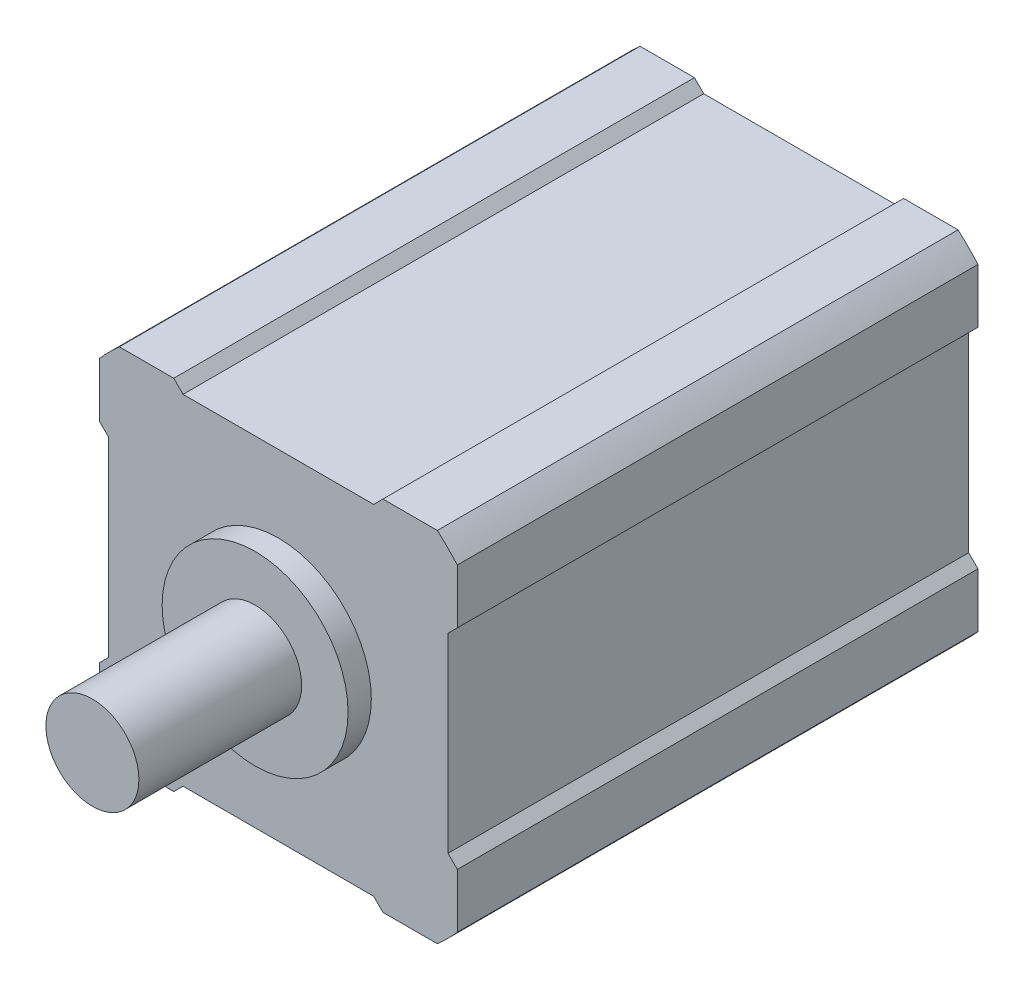
from build123d import *

# Parameters (mm, degrees)
SKETCH1_W           = 77
SKETCH1_H           = 77
EXTRUDE1_DEPTH      = 112
SKETCH3_R           = 58.910335971
SKETCH3_R_2         = 51.5
EXTRUDE3_DEPTH      = 125.533128123
EXTRUDE7_DEPTH      = 125.533128123
SKETCH2_R           = 10
EXTRUDE10_DEPTH     = 80
CIRPATTERN3_COUNT   = 4
EXTRUDE13_START     = 5
SKETCH11_R          = 20
SKETCH11_R_2        = 10
EXTRUDE13_DEPTH     = 5
BOSS_EXTRUDE1_START = 120
SKETCH12_R          = 10
BOSS_EXTRUDE1_DEPTH = 120
SCALE1_SCALE        = 0.55


with BuildPart() as part:
    # Sketch1 → Extrude1 (new body)
    with BuildSketch(Plane.XY):
        Rectangle(SKETCH1_W, SKETCH1_H)
    extrude(amount=EXTRUDE1_DEPTH)

    # Sketch3 → Extrude3 (cut, through all)
    with BuildSketch(Plane.XY.offset(112)):
        Circle(SKETCH3_R)
        Circle(SKETCH3_R_2, mode=Mode.SUBTRACT)
    extrude(amount=-EXTRUDE3_DEPTH, mode=Mode.SUBTRACT)

    # Sketch7 → Extrude7 (cut, through all)
    with BuildSketch(Plane.XY.offset(112)):
        Polygon((-22.5, 38.5), (22.5, 38.5), (20.5, 36.5), (-20.5, 36.5), align=None)
    extrude7 = extrude(amount=-EXTRUDE7_DEPTH, mode=Mode.SUBTRACT)

    # Sketch2 → Extrude10 (cut)
    with BuildSketch(Plane.XY.offset(112)):
        Circle(SKETCH2_R)
    extrude(amount=-EXTRUDE10_DEPTH, mode=Mode.SUBTRACT)

    # CirPattern3: Extrude7 ×4 about axis
    cirpattern3_axis = Axis((0, 0, 0), (0, 0, 1))
    for i in range(1, CIRPATTERN3_COUNT):
        add(extrude7.rotate(cirpattern3_axis, i * 360 / CIRPATTERN3_COUNT), mode=Mode.SUBTRACT)

    # Sketch11 → Extrude13 (add)
    with BuildSketch(Plane.XY.offset(112).offset(EXTRUDE13_START)):
        Circle(SKETCH11_R)
        Circle(SKETCH11_R_2, mode=Mode.SUBTRACT)
    extrude(amount=-EXTRUDE13_DEPTH)

    # Sketch12 → Boss-Extrude1 (add)
    with BuildSketch(Plane.XY.offset(32).offset(BOSS_EXTRUDE1_START)):
        Circle(SKETCH12_R)
    extrude(amount=-BOSS_EXTRUDE1_DEPTH)


with BuildPart() as part_1:
    # Scale1: scaled about (0, 0, 57.926521071)
    add(part.part.scale(SCALE1_SCALE).moved(Location((0, 0, 26.066934482))))


solid = part_1.part
